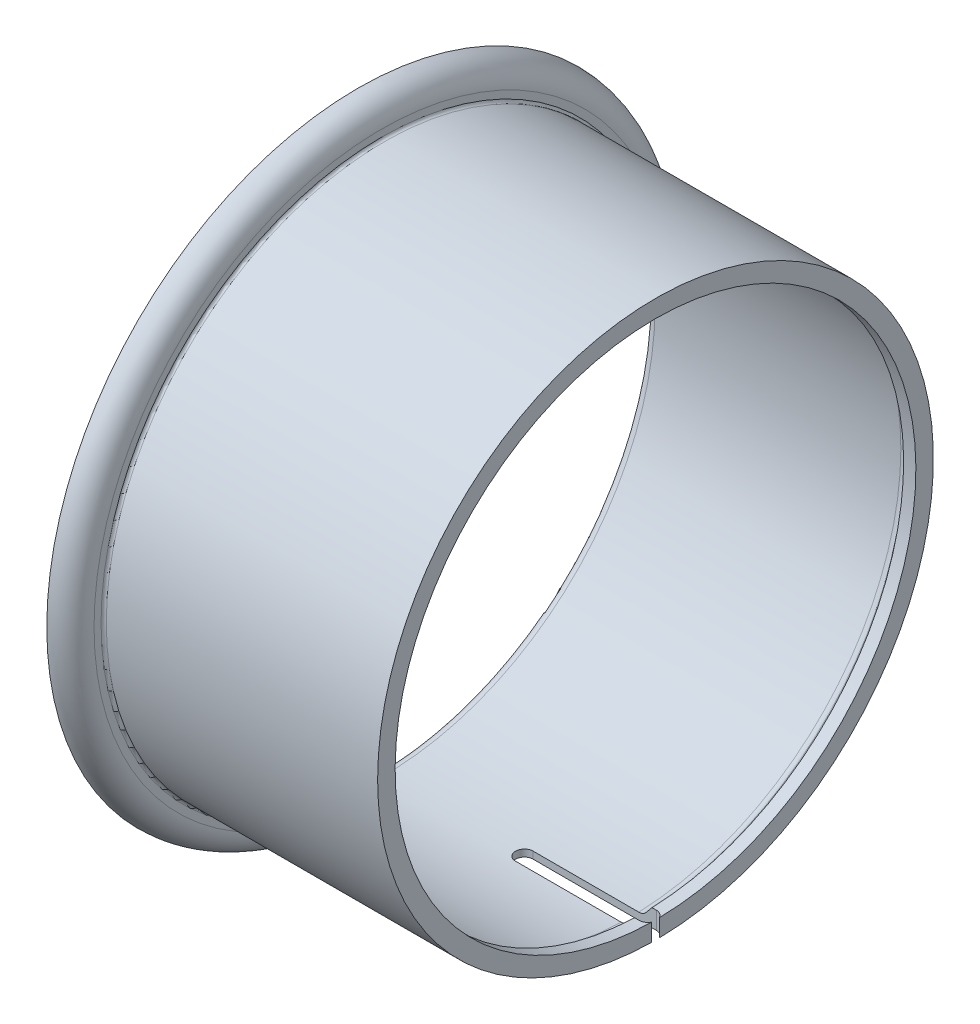
from build123d import *

# Parameters (mm, degrees)
FILLET_2_R          = 11
FILLET_3_R          = 3
CUT_EXTRUDE_3_DEPTH = 607.927096175


with BuildPart() as part:
    # 草图1 → 旋转1 (revolve)
    with BuildSketch(Plane.XY, mode=Mode.PRIVATE) as revolve_1_sk:
        with BuildLine():
            Line((19, 328.5), (19, 309.5))
            Line((19, 309.5), (316, 309.5))
            Line((316, 309.5), (326, 297.5))
            Line((326, 297.5), (340, 297.5))
            Line((340, 297.5), (340, 317.5))
            Line((340, 317.5), (27, 317.5))
            Line((27, 317.5), (27, 328.5))
            ThreePointArc((27, 328.5), (19.091883092, 347.591883092), (0, 355.5))
            Line((0, 355.5), (0, 347.5))
            ThreePointArc((0, 347.5), (13.435028843, 341.935028843), (19, 328.5))
        make_face()
    revolve(revolve_1_sk.sketch.rotate(Axis((-326.852669965, 0, 0), (1, 0, 0)), 90), axis=Axis((-326.852669965, 0, 0), (1, 0, 0)))

    # 圆角2
    fillet_2_edges = [part.edges().sort_by_distance(p)[0] for p in [
        (316, 0, -309.5),
        (19, 0, -309.5),
    ]]
    fillet(fillet_2_edges, radius=FILLET_2_R)

    # 圆角3
    fillet_3_edges = [part.edges().sort_by_distance(p)[0] for p in [
        (27, 0, -317.5),
    ]]
    fillet(fillet_3_edges, radius=FILLET_3_R)

    # 草图2 → 切除-拉伸3 (cut, through all)
    with BuildSketch(Plane(origin=(0, 0, 0), x_dir=(1, 0, 0), z_dir=(0, 1, 0))):
        with BuildLine():
            Line((190, 10), (331, 10))
            ThreePointArc((331, 10), (341, 0), (331, -10))
            Line((331, -10), (190, -10))
            ThreePointArc((190, -10), (180, 0), (190, 10))
        make_face()
    extrude(amount=-CUT_EXTRUDE_3_DEPTH, mode=Mode.SUBTRACT)


solid = part.part
